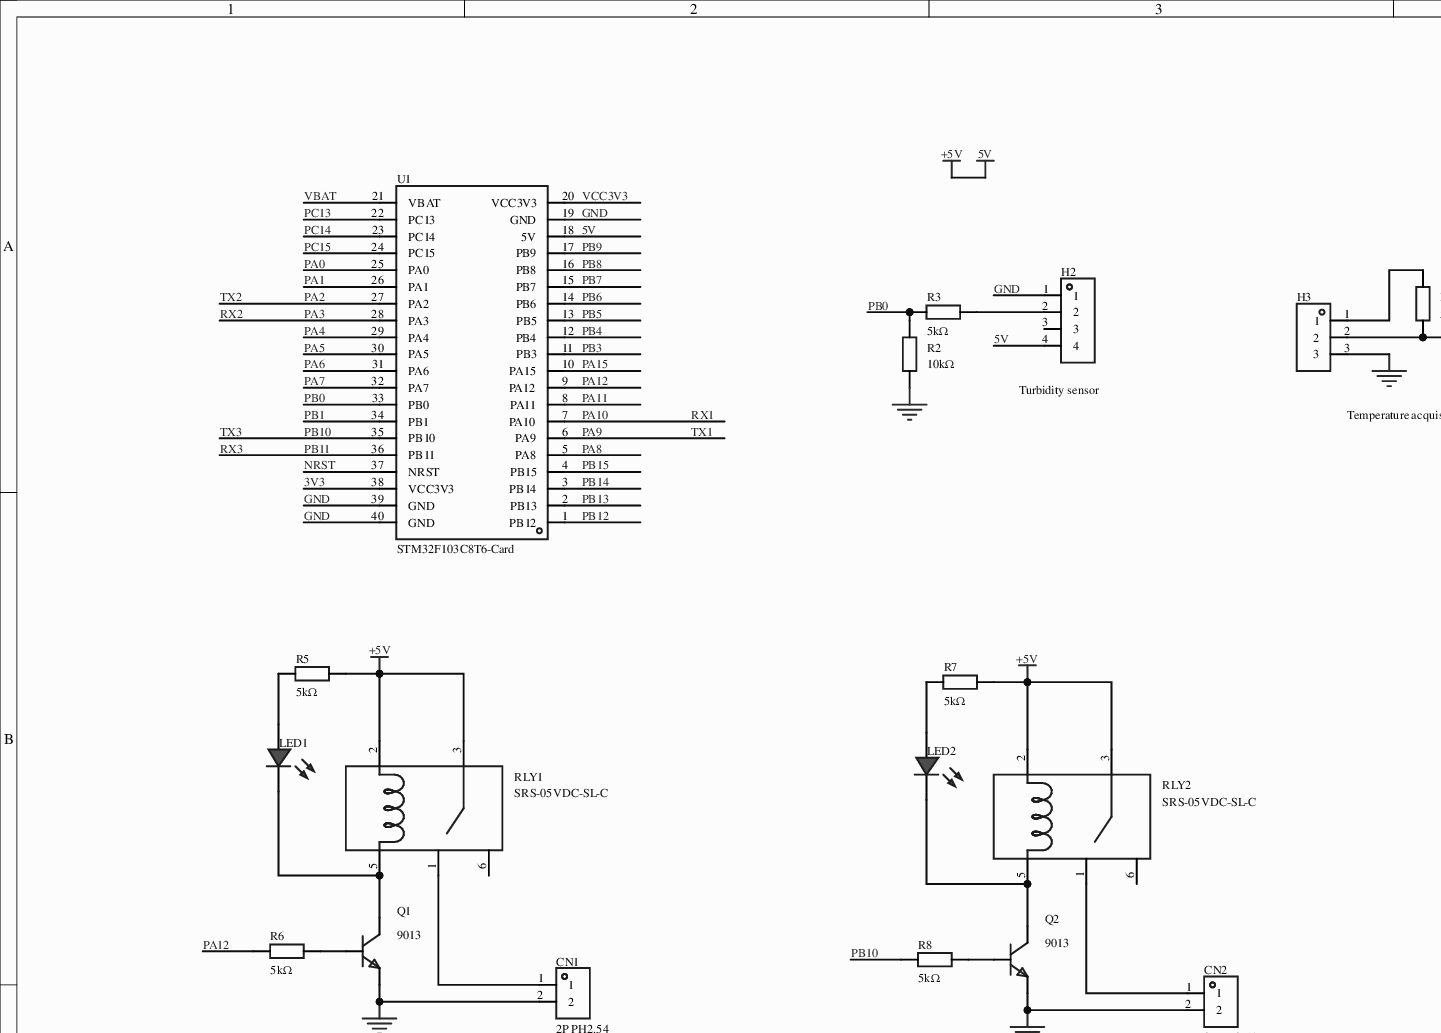
[diagram p0: MISC50991-3.schdoc, top left]
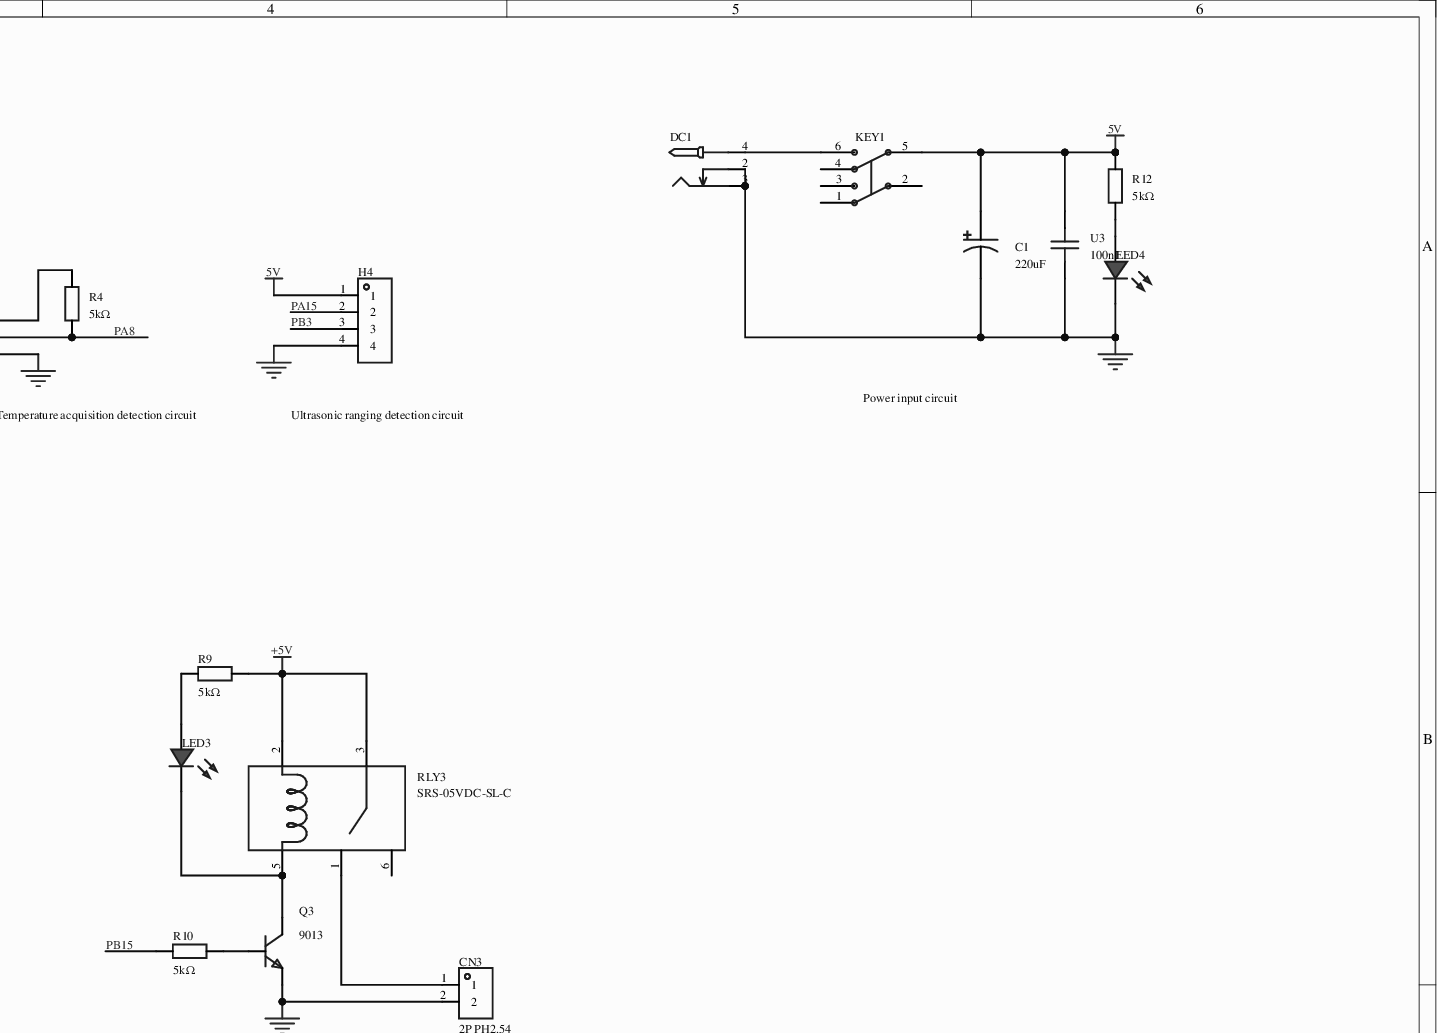
[diagram p1: MISC50991-3.schdoc, top right]
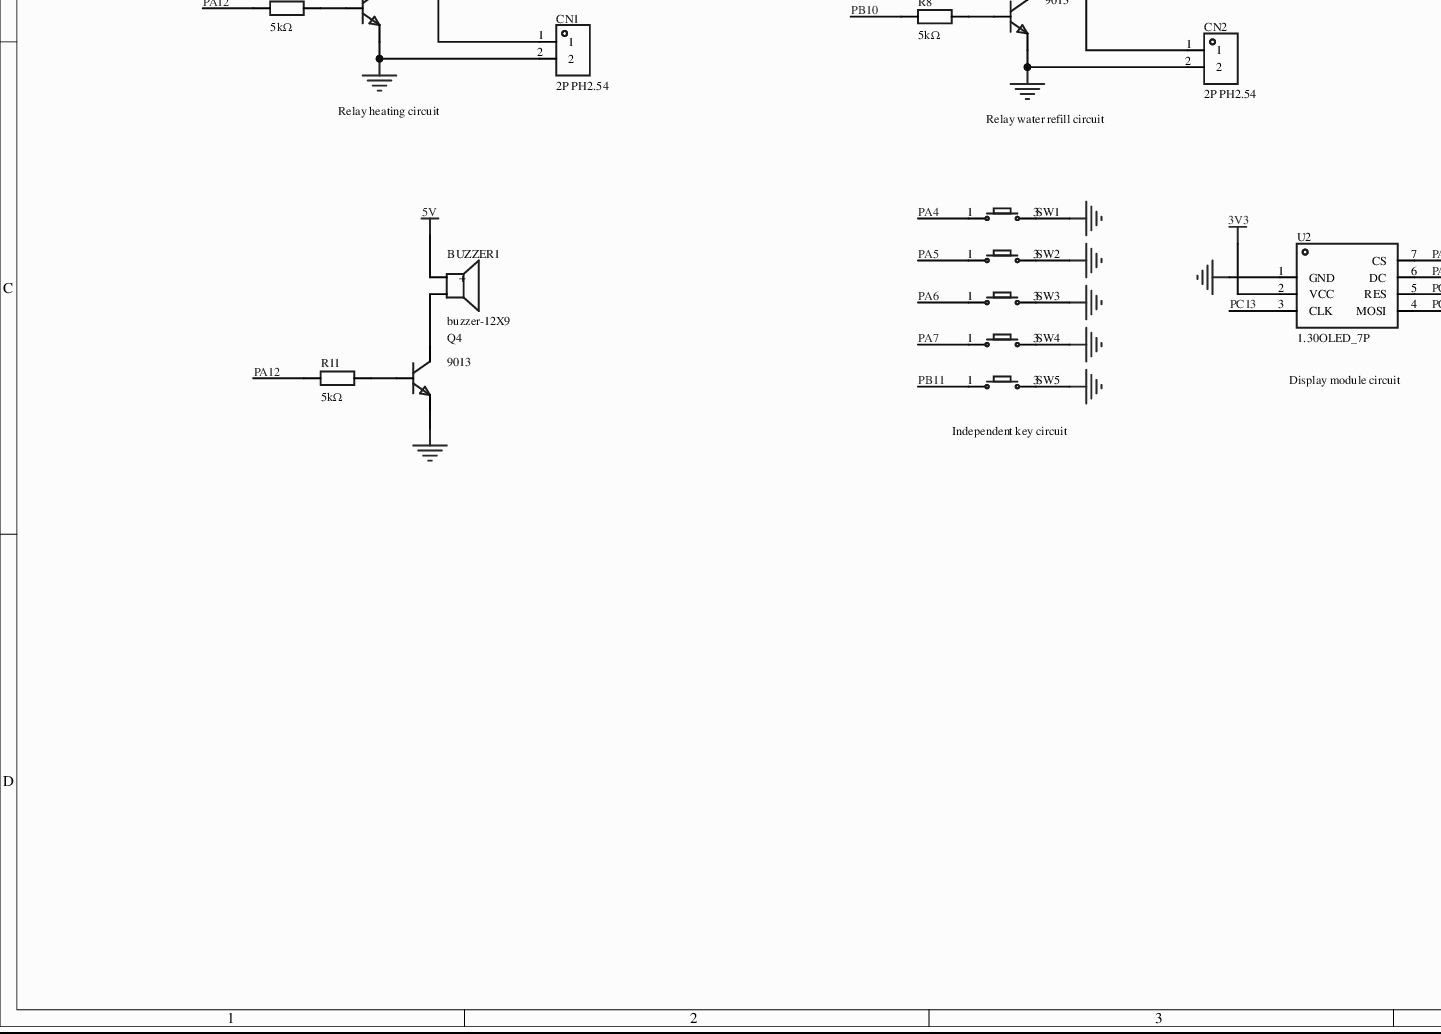
[diagram p2: MISC50991-3.schdoc, bottom left]
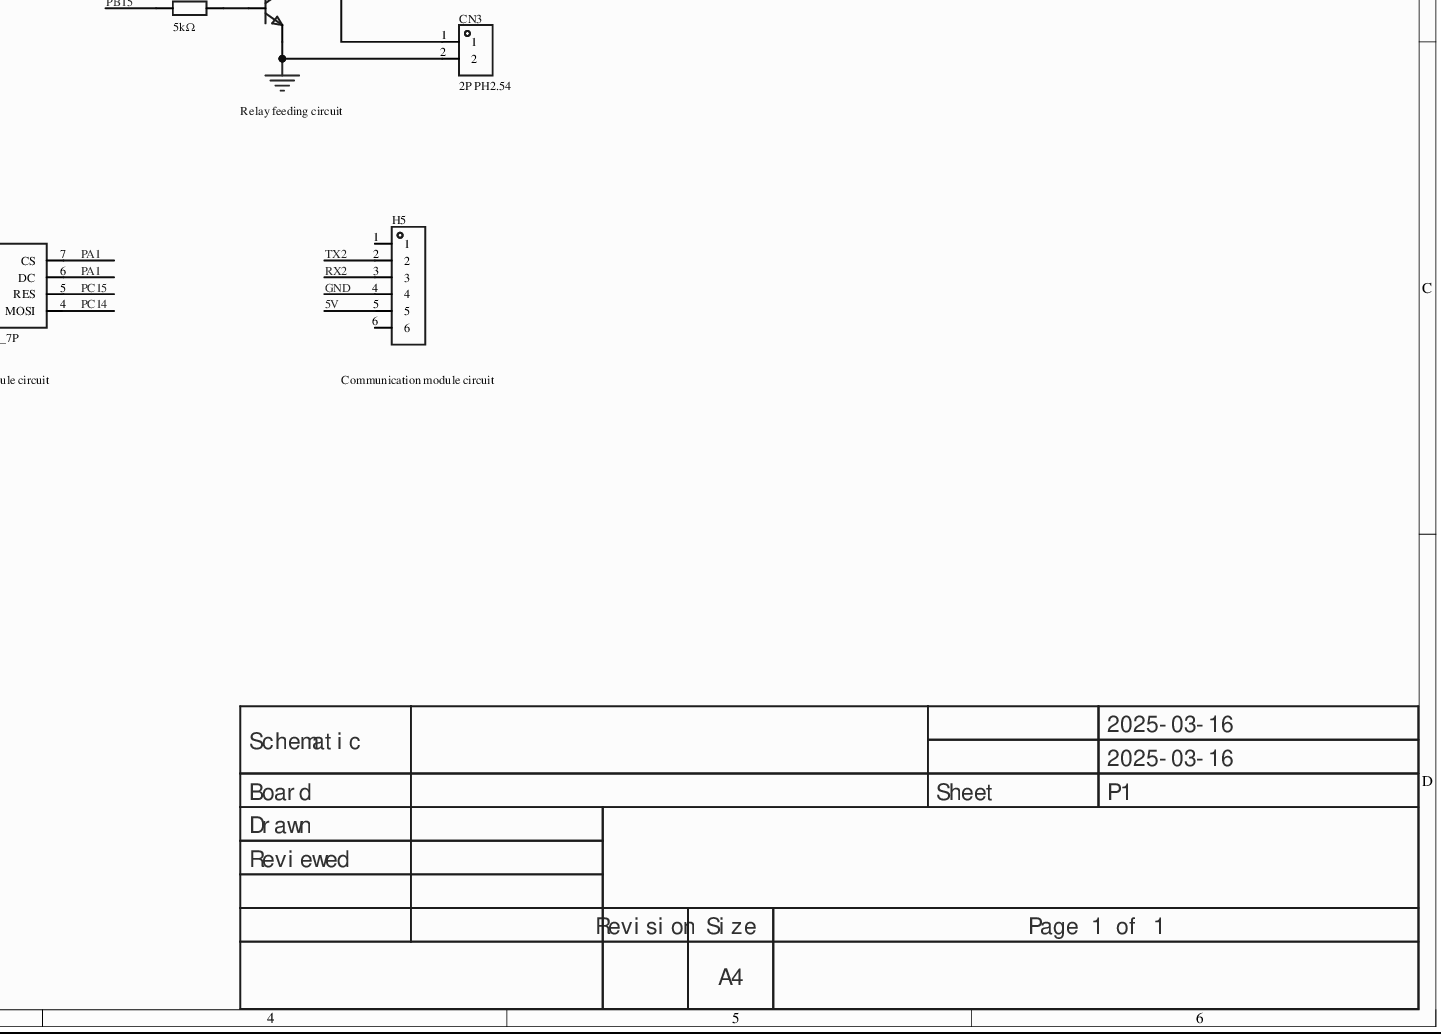
[diagram p3: MISC50991-3.schdoc, bottom right]
# Altium project MISC50991-2.PrjPcb
1 sheet, 41 parts. Net scope: global (net labels, ports and power ports of the same name join across sheets).
Board file: MISC50991.pcbdoc

## Sheet MISC50991-3.schdoc
size 420 x 297 mm; Version: V1.0; @Project Name: MISC50991; @Page Count: 1; @Update Date: 2025-03-16; @Create Date: 2025-03-16; @Schematic Name: MISC50991; @Page No: 1; @Create Time: 17:15:21; @Update Time: 17:42:28; @Board Name: MISC50991

### Parts
BUZZER1  buzzer-12X9  [BUZ-TH_BD12.0-P7.60-D0.6-FD]
C1  220uF  [CAP-TH_BD6.3-P2.50-D1.0-FD]
CN1  2P PH2.54  [CONN-TH_2P-P2.54_HDR2]
CN2  2P PH2.54  [CONN-TH_2P-P2.54_HDR2]
CN3  2P PH2.54  [CONN-TH_2P-P2.54_HDR2]
DC1  (no value)  [DC-2.0]
H2  (no value)  [HDR-TH_4P-P2.54-V-F]
H3  (no value)  [HDR-TH_3P-P2.54-V-F]
H4  (no value)  [HDR-TH_4P-P2.54-V-F]
H5  (no value)  [HDR-TH_6P-P2.54-V-F]
KEY1  Non-latching switch 8.5×8.5 silent  [SW-TH_6P-L8.5-W8.5-P2.54]  (value not drawn)
LED1  (no value)  [LED-TH_5mm]
LED2  (no value)  [LED-TH_5mm]
LED3  (no value)  [LED-TH_5mm]
LED4  (no value)  [LED-TH_5mm]
Q1  9013  [TO-92-3_L4.8-W3.7-P2.54-R]
Q2  9013  [TO-92-3_L4.8-W3.7-P2.54-R]
Q3  9013  [TO-92-3_L4.8-W3.7-P2.54-R]
Q4  9013  [TO-92-3_L4.8-W3.7-P2.54-R]
R2  10kΩ  [Res_1/4W]
R3  5kΩ  [Res_1/4W]
R4  5kΩ  [Res_1/4W]
R5  5kΩ  [Res_1/4W]
R6  5kΩ  [Res_1/4W]
R7  5kΩ  [Res_1/4W]
R8  5kΩ  [Res_1/4W]
R9  5kΩ  [Res_1/4W]
R10  5kΩ  [Res_1/4W]
R11  5kΩ  [Res_1/4W]
R12  5kΩ  [Res_1/4W]
RLY1  SRS-05VDC-SL-C  [RELAY-TH_SRS-05VDC-SL-C]
RLY2  SRS-05VDC-SL-C  [RELAY-TH_SRS-05VDC-SL-C]
RLY3  SRS-05VDC-SL-C  [RELAY-TH_SRS-05VDC-SL-C]
SW1  (no value)  [SW-TH_4P-L6.0-W6.0-P4.50-LS6.5]
SW2  (no value)  [SW-TH_4P-L6.0-W6.0-P4.50-LS6.5]
SW3  (no value)  [SW-TH_4P-L6.0-W6.0-P4.50-LS6.5]
SW4  (no value)  [SW-TH_4P-L6.0-W6.0-P4.50-LS6.5]
SW5  (no value)  [SW-TH_4P-L6.0-W6.0-P4.50-LS6.5]
U1  STM32F103C8T6-Card  [CONN-TH_L53.3-W22.9_STM32F103C8T6-CARD]
U2  1.30OLED_7P  [LCD-TH_7P-P2.54_1.30OLED_7P]
U3  100nF  [CAP-TH_L5.0-W2.5-P5.00-D1.0]

### Nets
3V3: U1.38(VCC3V3) U2.2(VCC)
+5V: BUZZER1.1(+) C1.1 H2.4 H4.1 H5.5 KEY1.5 R5.2 R7.2 R9.2 R12.2 RLY1.2 RLY1.3 RLY2.2 RLY2.3 RLY3.2 RLY3.3 U1.18(5V) U3.1  [also labelled 5V]
GND: C1.2 CN1.2 CN2.2 CN3.2 DC1.2 DC1.3 H2.1 H3.3 H4.4 H5.4 LED4.2(A) Q1.3(E) Q2.3(E) Q3.3(E) Q4.3(E) R2.1 SW1.3 SW2.3 SW3.3 SW4.3 SW5.3 U1.19(GND) U1.39(GND) U1.40(GND) U2.1(GND) U3.2
NRST: U1.37(NRST)
PA0: U1.25(PA0)
PA1: U1.26(PA1) U2.6(DC) U2.7(CS)
PA2: H5.2 U1.27(PA2)  [also labelled TX2]
PA3: H5.3 U1.28(PA3)  [also labelled RX2]
PA4: SW1.1 U1.29(PA4)
PA5: SW2.1 U1.30(PA5)
PA6: SW3.1 U1.31(PA6)
PA7: SW4.1 U1.32(PA7)
PA8: H3.2 R4.1 U1.5(PA8)
PA9: U1.6(PA9)  [also labelled TX1]
PA10: U1.7(PA10)  [also labelled RX1]
PA11: U1.8(PA11)
PA12: R6.1 R11.1 U1.9(PA12)
PA15: H4.2 U1.10(PA15)
PB0: R2.2 R3.1 U1.33(PB0)
PB1: U1.34(PB1)
PB3: H4.3 U1.11(PB3)
PB4: U1.12(PB4)
PB5: U1.13(PB5)
PB6: U1.14(PB6)
PB7: U1.15(PB7)
PB8: U1.16(PB8)
PB9: U1.17(PB9)
PB10: R8.1 U1.35(PB10)  [also labelled TX3]
PB11: SW5.1 U1.36(PB11)  [also labelled RX3]
PB12: U1.1(PB12)
PB13: U1.2(PB13)
PB14: U1.3(PB14)
PB15: R10.1 U1.4(PB15)
PC13: U1.22(PC13) U2.3(CLK)
PC14: U1.23(PC14) U2.4(MOSI)
PC15: U1.24(PC15) U2.5(RES)
VBAT: U1.21(VBAT)
VCC3V3: U1.20(VCC3V3)
NetBUZZER1_2: BUZZER1.2 Q4.1(C)
NetCN1_1: CN1.1 RLY1.1
NetCN2_1: CN2.1 RLY2.1
NetCN3_1: CN3.1 RLY3.1
NetDC1_4: DC1.4 KEY1.6
NetH2_2: H2.2 R3.2
NetH3_1: H3.1 R4.2
NetLED1_1: LED1.1(C) R5.1
NetLED1_2: LED1.2(A) Q1.1(C) RLY1.5
NetLED2_1: LED2.1(C) R7.1
NetLED2_2: LED2.2(A) Q2.1(C) RLY2.5
NetLED3_1: LED3.1(C) R9.1
NetLED3_2: LED3.2(A) Q3.1(C) RLY3.5
NetLED4_1: LED4.1(C) R12.1
NetQ1_2: Q1.2(B) R6.2
NetQ2_2: Q2.2(B) R8.2
NetQ3_2: Q3.2(B) R10.2
NetQ4_2: Q4.2(B) R11.2

Not connected (* = marked no-connect by the designer): H2 3*; H5 1 6; KEY1 1 2 3 4; RLY1 6; RLY2 6; RLY3 6

### Notes on the sheet
- (near H2) Turbidity sensor
- Power input circuit
- Temperature acquisition detection circuit
- (near H4) Ultrasonic ranging detection circuit
- Relay heating circuit
- Relay water refill circuit
- Relay feeding circuit
- (near U2) Display module circuit
- (near H5) Communication module circuit
- (near SW5) Independent key circuit
- 2025-03-16
- Schematic
- Board
- Sheet
- P1
- Drawn
- Reviewed
- Revision
- Size
- A4
- Page 1 of 1

### Library data of the parts
BUZZER1 = buzzer-12X9: AddInBom: yes; ModelId: 16ab50e14c5b4f2c986c135bdba60e37; ModelName: BUZ-TH_D12.0-H9.5-P7.60; ModelTransform: 472.44,472.176,0,90,0,0,-0.787,0,-177.165; Symbol: BUZZER-12X9; Device: buzzer-12X9; LCSC Part Name: buzzer-12X9; SupplierPart: C9900016920; ManufacturerPart: buzzer-12X9; Supplier Footprint: BUZZER_SMT_9650B; JLCPCB Part Class: Extended library; Supplier: LCSC; ConvertToPcb: yes; FootprintName: BUZ-TH_BD12.0-P7.60-D0.6-FD
C1 = SS2271AMD052RB: Capacitance: 220uF; Tolerance: ±20%; Rated voltage: 10V; Ripple current: -; ESR: -;; Manufacturer: Xunda(讯达); AddInBom: yes; ModelId: 0a4db4bf24b443b3be4905be97ff10c5; ModelTransform: 248.4247,247.99777,0,0,0,0,0,0,-137.795; φD: 6.3mm; L: 5mm; Lifetime @ Temp: 2000hrs@105℃; Symbol: SS2271AMD052RB; Device: SS2271AMD052RB; LCSC Part Name: 220uF ±20% 10V; SupplierPart: C399137; ManufacturerPart: SS2271AMD052RB; Supplier Footprint: 插件,D6.3xL5mm; JLCPCB Part Class: Extended library; Datasheet: https://atta.szlcsc.com/upload/public/pdf/source/20190625/C399162_74BDC4DC8CD273727ECFDC61FC0FB83B.pdf; Supplier: LCSC; ConvertToPcb: yes; FootprintName: CAP-TH_BD6.3-P2.50-D1.0-FD; ModelName: CAP-TH_BD6.3-P2.50-D1.0-FD; Value: 220uF; Rated Voltage: 10V; Ripple Current: -; Equivalent Series Resistance(ESR): -; Lead Spacing: 2.5mm
CN1-CN3 = 2P PH2.54: AddInBom: yes; ModelId: d73fc62480cf45898e8bab8f216da528; ModelTransform: 295.275,224.409,0,180,0,0,0,17.717,-118.11; Symbol: 2P PH2.54; Device: 2P PH2.54; LCSC Part Name: 2P PH2.54; SupplierPart: C9900006197; ManufacturerPart: 2P PH2.54; Supplier Footprint: PH2.54; Supplier: LCSC; ConvertToPcb: yes; FootprintName: CONN-TH_2P-P2.54_HDR2; ModelName: CONN-TH_2P-P2.54_HDR2
DC1 = DC-005_2.0: ConvertToPcb: yes; SymbolName: DC power jack; ModelId: f5f20b8a2308479b936ba3c2698865bb0819f05c4eef4c71ace90d822a990e87; ModelName: DC-IN-TH_DC-5520-1; ModelTransform: 372.05,551.18,582.68,90,0,0,137.8,0,-149.61; Device: DC-005_2.0; AddInBom: yes; Supplier Footprint: 插件; FootprintName: DC-2.0
H2 H4 = HDR-F_2.54_1x4P: Symbol: 2.54-1*4P female; ConvertToPcb: yes; ModelId: d187812051054f85879fcaa51a310d8e; ModelTransform: 419.6842,98.464,0,0,0,0,0,0,-118.11; Device: HDR-F_2.54_1x4P; AddInBom: yes; SupplierPart: C2718488; Supplier Footprint: 插件; FootprintName: HDR-TH_4P-P2.54-V-F; ModelName: HDR-TH_4P-P2.54-V-F
H3 = HDR-F_2.54_1x3P: Symbol: PM254V-11-03-H85; ConvertToPcb: yes; ModelId: f3b3cc5aae9641bf9e56fc160cef875b; ModelName: HDR2.54-F-LI-1X3P; ModelTransform: 299.9994,100,0,0,0,0,0,0,-118.11; Device: HDR-F_2.54_1x3P; AddInBom: yes; SupplierPart: C541850; Supplier Footprint: 插件; FootprintName: HDR-TH_3P-P2.54-V-F
H5 = HDR-F_2.54_1x6P: Symbol: Header-Female-2.54_1x6; ConvertToPcb: yes; ModelId: 0f5bcf94dcda47d085f24cdca1696fe9; ModelTransform: 619.684,94.488,0,0,0,0,0,0,-125.984; Device: HDR-F_2.54_1x6P; AddInBom: yes; SupplierPart: C40877; Supplier Footprint: 插件; FootprintName: HDR-TH_6P-P2.54-V-F; ModelName: HDR-TH_6P-P2.54-V-F
KEY1 = 无自锁开关 8.5×8.5 无声: 6 pins, 8.5×8.5; Symbol: No self-locking switch 8.5×8.5 silent; AddInBom: yes; ModelId: 4c72b3966b92446eb355e1bd0fb4f880; ModelTransform: 342.519,334.645,0,180,0,0,0,0,-137.795; Device: Non-latching switch 8.5×8.5 silent; LCSC Part Name: 无自锁开关 8.5×8.5  无声; SupplierPart: C26228; ManufacturerPart: 无自锁开关 8.5×8.5 无声; Supplier Footprint: 插件; JLCPCB Part Class: Extended library; Supplier: LCSC; ConvertToPcb: yes; FootprintName: SW-TH_6P-L8.5-W8.5-P2.54; ModelName: SW-TH_6P-L8.5-W8.5-P2.54
LED1-LED4 = LED_TH-R_5mm: ConvertToPcb: yes; ModelId: fe9cea1bdf7642cd8d9a5077ed0e2b58; ModelName: LED-TH_BD5.9-P2.54-RD_RED; ModelTransform: 222.16,238.98,581.81,180,0,0,-6,0,-220; Symbol: LED_TH-R; Device: LED_TH-R_5mm; AddInBom: yes; FootprintName: LED-TH_5mm; Supplier Footprint: 插件
Q1-Q4 = 9013: Transistor type: NPN; Collector current (Ic): 500mA; Collector-emitter breakdown voltage (Vceo): 20V; Power (Pd): 625mW;; Manufacturer: BLUE ROCKET(蓝箭); AddInBom: yes; ModelId: 0fb83455cf6d479b95862acdd73b6eef; ModelName: TO-92-3_L4.8-W3.7-H7.7-P2.54-R; ModelTransform: 218.897,161.417,0,180,0,0,0,13.78,-433.071; Collector Cut-Off Current (Icbo): 100nA; Symbol: 9013; Device: 9013; LCSC Part Name: NPN 电流:500mA 耐压:20V; SupplierPart: C3037603; ManufacturerPart: 9013; Supplier Footprint: TO-92-2.54mm; Supplier: LCSC; ConvertToPcb: yes; FootprintName: TO-92-3_L4.8-W3.7-P2.54-R; Transistor Type: NPN; Collector Current (Ic): 500mA; Collector-Emitter Breakdown Voltage (Vceo): 20V; Power Dissipation (Pd): 625mW
R2-R12 = Res_AXIAL-1/4W: AddInBom: yes; SymbolName: Resistor; ModelId: 463263665006444ab7a47bd11b0cf956; ModelName: RES-TH_BD2.4-L6.3-P10.30-D0.6; ModelTransform: 427.165,94.32816,0,0,0,0,0,0,-196.85; Device: Res_AXIAL-1/4W; Supplier Footprint: 轴向引线; ConvertToPcb: yes; FootprintName: Res_1/4W
  R2: Value: 10kΩ
  R3-R12: Value: 5kΩ
RLY1-RLY3 = SRS-05VDC-SL-C: AddInBom: yes; ModelId: a12ba931fcd442a78bfd92976a1f634e; ModelTransform: 622.046,425.5897,0,180,0,0,-7.874,0,-118.11; Symbol: SRS-05VDC-SL-C; Device: SRS-05VDC-SL-C; LCSC Part Name: SRS-05VDC-SL-C; SupplierPart: C9900062817; ManufacturerPart: SRS-05VDC-SL-C; Supplier Footprint: 插件; Supplier: LCSC; ConvertToPcb: yes; FootprintName: RELAY-TH_SRS-05VDC-SL-C; ModelName: RELAY-TH_SRS-05VDC-SL-C
SW1-SW5 = Key_TH_6x6x6: Contact current: 50mA; Rated voltage (DC): 12V; Insulation resistance: 100MΩ; Circuit structure: SPST; Mounting: through-hole; Button shape: round button; Button/cap colour: black; Actuation force: 260gf@±30gf; Operating temperature: -25℃~+70℃; Pin style: PC pin; Switch length: 6mm; Switch width: 6mm; Switch height: 6mm; With bracket: no;; Symbol: Tactile switch; ConvertToPcb: yes; ModelId: 20eee248bc684ccd8cbdbb1d0d91ec6f; ModelName: SW-TH_4P-L6.0-W6.0-H5.0-LS6.5-P4.50; ModelTransform: 236.22,323.03,0,90,0,0,0,0,-137.795; Device: Key_TH_6x6x6; AddInBom: yes; SupplierPart: C2837516; Supplier Footprint: 插件; FootprintName: SW-TH_4P-L6.0-W6.0-P4.50-LS6.5
U1 = STM32F103C8T6-Card: AddInBom: yes; Symbol: STM32F103C8T6-CARD; Device: STM32F103C8T6-Card; LCSC Part Name: STM32F103C8T6-Card; SupplierPart: C9900077949; ManufacturerPart: STM32F103C8T6-Card; Supplier Footprint: 插件; Supplier: LCSC; ConvertToPcb: yes; FootprintName: CONN-TH_L53.3-W22.9_STM32F103C8T6-CARD
U2 = 1.30OLED_7P: AddInBom: yes; ModelId: f23c42c7ec37494aa45fade310250424; ModelTransform: 1392.911,1319.28862,0,0,0,0,-0.984,-575.786,-196.85; Symbol: 1.30OLED_7P; Device: 1.30OLED_7P; LCSC Part Name: 1.30OLED_7P; SupplierPart: C9900102405; ManufacturerPart: 1.30OLED_7P; Supplier Footprint: 4PQT130LWH30PG01S7V11_1.30OLED; JLCPCB Part Class: Extended library; Supplier: LCSC; ConvertToPcb: yes; FootprintName: LCD-TH_7P-P2.54_1.30OLED_7P; ModelName: LCD-TH_7P-P2.54_1.30OLED_7P
U3 = 100nF: Symbol: 100NF_C9900015256; AddInBom: yes; ModelId: 08e3d7481fc7486bb1b263873f51e1e1; ModelName: CAP-TH_BD5.0-W2.5-P5.08; ModelTransform: 224.652,98.425,0,0,0,0,-0.005,0,-137.795; Device: 100nF; LCSC Part Name: 100nF; SupplierPart: C9900015256; ManufacturerPart: 100nF; Supplier Footprint: CAP-TH_L5.0-W2.5-P5.00-D1.0; Supplier: LCSC; ConvertToPcb: yes; FootprintName: CAP-TH_L5.0-W2.5-P5.00-D1.0